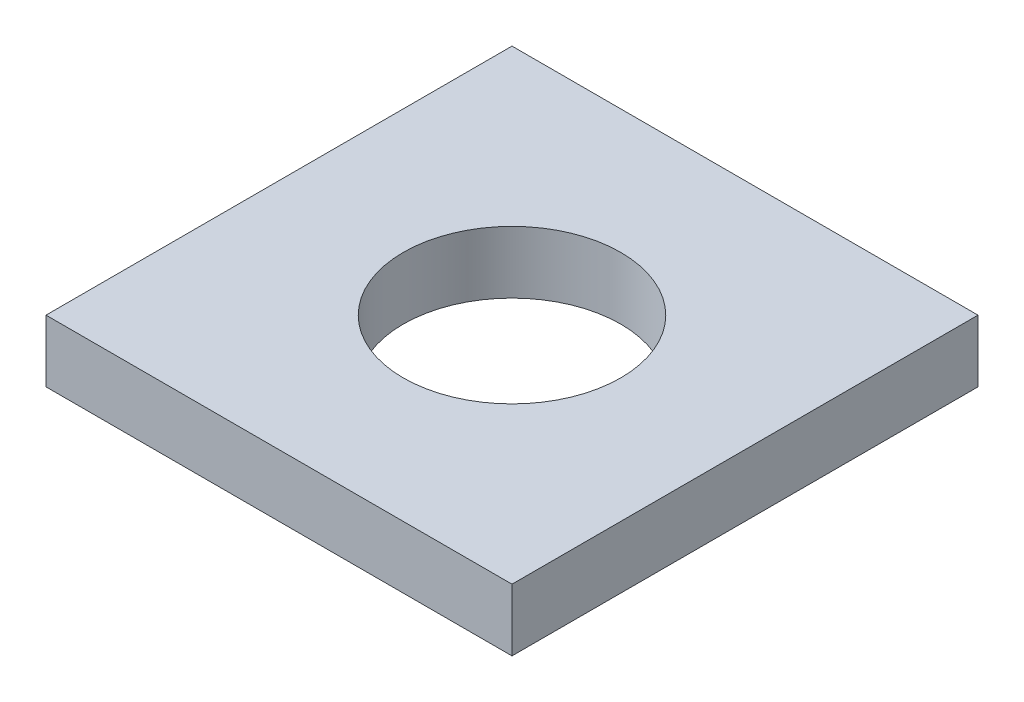
from build123d import *

# Parameters (mm, degrees)
SKETCH1_W           = 30
SKETCH1_H           = 30
BOSS_EXTRUDE1_DEPTH = 4
SKETCH3_R           = 7
CUT_EXTRUDE2_DEPTH  = 43.614551505


with BuildPart() as part:
    # Sketch1 → Boss-Extrude1 (new body)
    with BuildSketch(Plane(origin=(0, 0, 0), x_dir=(1, 0, 0), z_dir=(0, 1, 0))):
        with Locations((15, -15)):
            Rectangle(SKETCH1_W, SKETCH1_H)
    extrude(amount=BOSS_EXTRUDE1_DEPTH)

    # Sketch3 → Cut-Extrude2 (cut, through all)
    with BuildSketch(Plane(origin=(0, 4, 0), x_dir=(1, 0, 0), z_dir=(0, 1, 0))):
        with Locations(Location((15, -15, 0), (0, 0, 270))):
            Circle(SKETCH3_R)
    extrude(amount=-CUT_EXTRUDE2_DEPTH, mode=Mode.SUBTRACT)


solid = part.part
